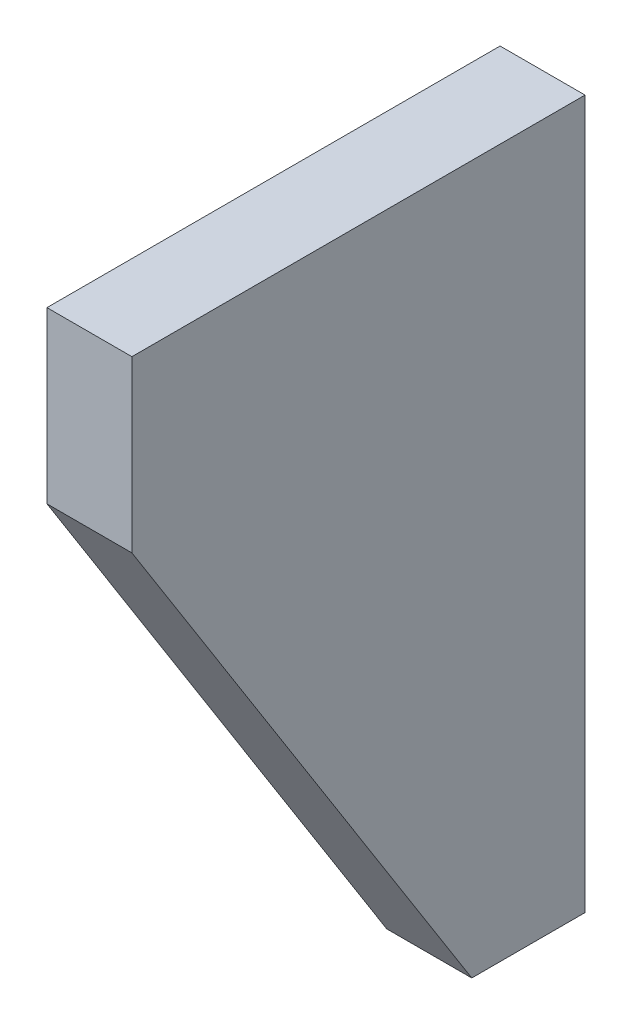
from build123d import *

# Parameters (mm, degrees)
BOSS_EXTRUDE1_DEPTH = 7.5


with BuildPart() as part:
    # Sketch1 → Boss-Extrude1 (new, symmetric)
    with BuildSketch(Plane(origin=(0, 0, 0), x_dir=(0, 0, -1), z_dir=(1, 0, 0))):
        Polygon((0, 0), (0, 125), (-80, 125), (-80, 95), (-20, 0), align=None)
    extrude(amount=BOSS_EXTRUDE1_DEPTH, both=True)


solid = part.part
